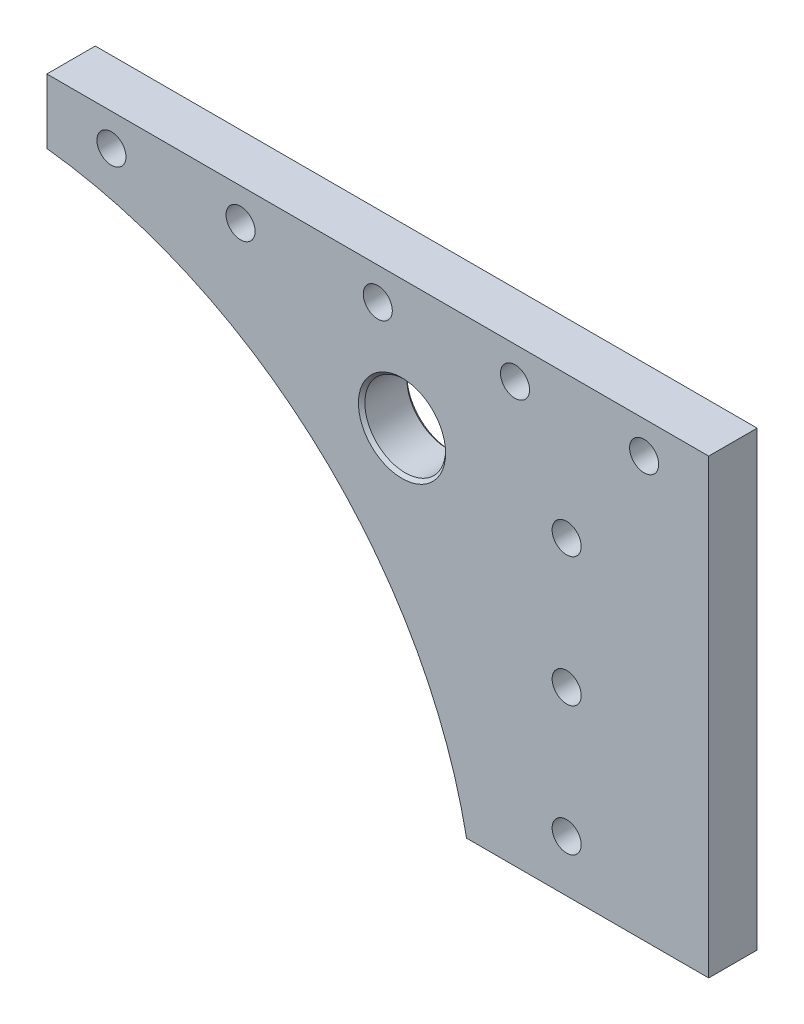
SolidWorks part; units mm, degrees
material "Q235A"
ref_plane "前视基准面" through (0, 0, 0) normal (0, 0, 1) x (1, 0, 0)
ref_plane "上视基准面" through (0, 0, 0) normal (0, 1, 0) x (1, 0, 0)
ref_plane "右视基准面" through (0, 0, 0) normal (1, 0, 0) x (0, 0, -1)
sketch "草图1" plane through (0, 0, 0) normal (0, 0, 1) x (1, 0, 0)
  line L0 (0, 0) -> (205, 0)
  line L1 (205, 0) -> (205, -140)
  line L2 (0, 0) -> (0, -20)
  line L3 (0, -20) -> (130, -140)
  line L4 (130, -140) -> (205, -140)
  dimension "D1" = 20
  dimension "D2" = 205
  dimension "D3" = 130
  dimension "D4" = 140
extrude "凸台-拉伸1" add sketch "草图1" along normal mid plane 15
sketch "草图2" plane through (0, 0, 7.5) normal (0, 0, 1) x (1, 0, 0)
  line L0 (0, -20) -> (130, -140) construction
  line L1 (27.0833, -45) -> (75, -45)
  line L2 (27.0833, -45) -> (27.0833, -89.2308)
  line L3 (27.0833, -89.2308) -> (75, -89.2308)
  line L4 (75, -45) -> (75, -89.2308)
  line L5 (0, 0) -> (0, -20) construction
  line L6 (205, 0) -> (0, 0) construction
  dimension "D1" = 75
  dimension "D2" = 45
extrude "切除-拉伸1" [suppressed] cut sketch "草图2" against normal through all
hole_wizard "M8 六角凹头螺钉的柱形沉头孔2" positions "草图5" profile "草图6" counterbore size "M8" standard "ISO" end condition through all
sketch "草图5" plane through (0, 0, -7.5) normal (0, 0, 1) x (1, 0, 0)
  line L2 (205, 0) -> (0, 0) construction
  point P0 (20, -10)
  point P3 (60, -10)
  point P6 (60, -10)
  point P8 (102.5, -10)
  point P11 (145, -10)
  point P15 (161, -44)
  point P18 (161, -84)
  point P21 (161, -124)
  point P43 (185, -10)
  dimension "D3" = 141
  dimension "D6" = 44
  dimension "D7" = 84
  dimension "D8" = 124
sketch "草图6" plane through (20, -10, -7.5) normal (1, 0, 0) x (0, 1, 0)
  line L0 (0, 0) -> (0, 15)
  line L1 (0, 15) -> (4.5, 15)
  line L3 (4.5, 15) -> (4.5, 8.6)
  line L4 (4.5, 8.6) -> (7.5, 8.6)
  line L5 (7.5, 8.6) -> (7.5, 0)
  line L7 (7.5, 0) -> (0, 0)
  line L11 (0, -6.35) -> (0, 107.95) construction
  dimension "通孔孔直径" = 9
  dimension "通孔孔深度" = 15
  dimension "柱形沉头孔直径" = 15
  dimension "柱形沉头孔深度" = 8.6
hole_wizard "M5 螺纹孔1" positions "草图7" profile "草图8" tap size "M5" standard "ISO"
sketch "草图7" plane through (0, 0, -7.5) normal (0, 0, 1) x (1, 0, 0)
  line L0 (20, -10) -> (60, -10)
  line L2 (102.5, -10) -> (145, -10)
  line L3 (161, -44) -> (161, -84)
  line L5 (161, -84) -> (161, -124)
  point P0 (40, -10)
  point P2 (123.75, -10)
  point P14 (161, -64)
  point P16 (161, -104)
cosmetic thread "孔螺蚊线1" parameters "D1"=10, "D2"=5
cosmetic thread "孔螺蚊线2" parameters "D1"=10, "D2"=5
sketch "草图8" plane through (40, -10, -7.5) normal (1, 0, 0) x (0, 1, 0)
  line L0 (0, 0) -> (0, 13.6618)
  line L1 (0, 13.6618) -> (2.1, 12.4)
  line L2 (2.1, 12.4) -> (2.1, 0)
  line L5 (2.1, 0) -> (0, 0)
  line L10 (0, 13.6618) -> (-2.1, 12.4) construction
  line L11 (0, -6.35) -> (0, 107.95) construction
  dimension "螺纹孔钻头直径" = 4.2
  dimension "螺纹孔钻头深度" = 12.4
  dimension "导头角度" = 118
cosmetic thread "孔螺蚊线3" parameters "D1"=10, "D2"=5
cosmetic thread "孔螺蚊线4" parameters "D1"=10, "D2"=5
sketch "草图9" plane through (0, 0, 7.5) normal (0, 0, 1) x (1, 0, 0)
  line L0 (0, -20) -> (130, -140) construction
  line L1 (57.5, -73.0769) -> (90, -73.0769)
  line L2 (57.5, -73.0769) -> (57.5, -103.0769)
  line L3 (57.5, -103.0769) -> (90, -103.0769)
  line L4 (90, -73.0769) -> (90, -103.0769)
  line L5 (0, 0) -> (0, -20) construction
  dimension "D1" = 30
  dimension "D2" = 90
extrude "切除-拉伸2" [suppressed] cut sketch "草图9" against normal through all
sketch "草图10" plane through (0, 0, 7.5) normal (0, 0, 1) x (1, 0, 0)
  line L1 (60.8333, -76.1538) -> (115, -76.1538)
  line L2 (60.8333, -76.1538) -> (60.8333, -126.1538)
  line L3 (60.8333, -126.1538) -> (115, -126.1538)
  line L4 (115, -76.1538) -> (115, -126.1538)
  line L7 (0, -20) -> (130, -140) construction
  line L9 (205, -140) -> (205, 0) construction
  dimension "D1" = 90
  dimension "D2" = 50
extrude "切除-拉伸3" [suppressed] cut sketch "草图10" against normal through all
fillet "圆角1" [suppressed] radius 10
sketch "草图11" plane through (0, 0, 7.5) normal (0, 0, 1) x (1, 0, 0)
  circle A0 centre (-17.1671, -169.0144) radius 150
  dimension "D1" = 300
extrude "切除-拉伸4" cut sketch "草图11" against normal through all
sketch "草图12" plane through (0, 0, -7.5) normal (0, 0, -1) x (-1, 0, 0)
  circle A0 centre (-110, -40) radius 12.5 construction
  circle A1 centre (-110, -40) radius 12.5
extrude "切除-拉伸5" cut sketch "草图12" against normal through all
chamfer "倒角1" distance 1 angle 45 2 edges at (97.5, -40, -7.5) (97.5, -40, 7.5)
